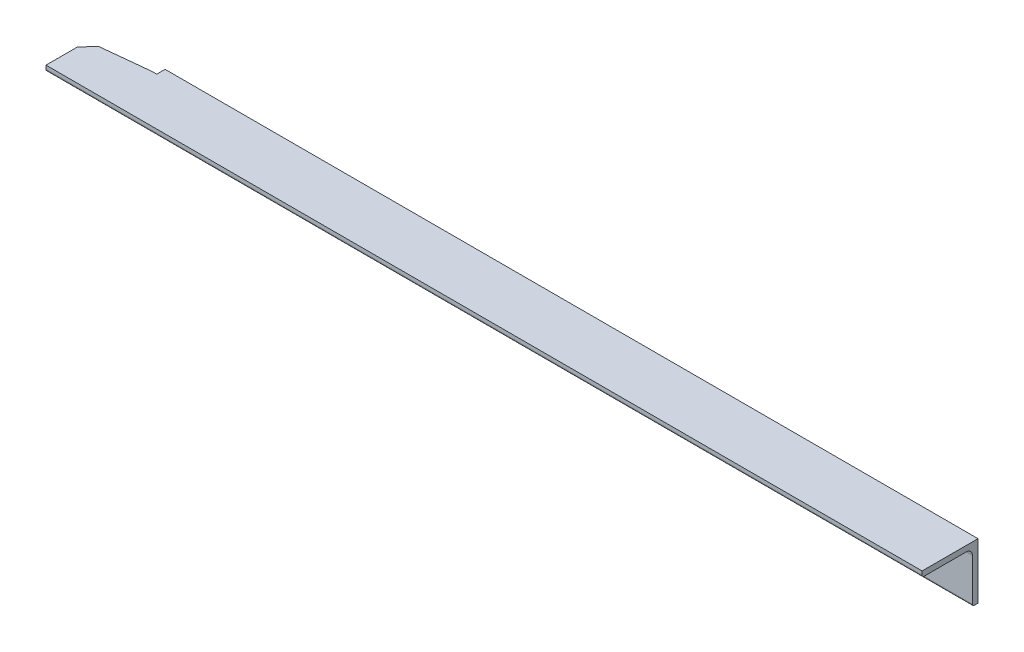
SolidWorks part; units mm, degrees
material "SPCC冷轧板喷塑"
ref_plane "前视基准面" through (0, 0, 0) normal (0, 0, 1) x (1, 0, 0)
ref_plane "上视基准面" through (0, 0, 0) normal (0, 1, 0) x (1, 0, 0)
ref_plane "右视基准面" through (0, 0, 0) normal (1, 0, 0) x (0, 0, -1)
other "Configuration Table"
sketch "草图1" plane through (0, 0, 0) normal (0, 0, 1) x (1, 0, 0)
  line L0 (391.75, 0) -> (-391.75, 0)
  point P4 (0, 0)
  dimension "D1" = 783.5
other "Gbt706-2008 热轧等边角钢 050×5(1)"
ref_plane "基准面1" through (391.75, 0, 0) normal (-1, 0, 0) x (0, -1, 0)
sketch "Sketch1" plane through (391.75, 0, 0) normal (-1, 0, 0) x (0, -1, 0)
  line L0 (0, 0) -> (0, 50)
  line L1 (0, 25) -> (5, 25) construction
  line L2 (5, 48.3333) -> (5, 10.5)
  line L3 (10.5, 5) -> (48.3333, 5)
  line L4 (25, 5) -> (25, 0) construction
  line L5 (50, 0) -> (0, 0)
  line L6 (0, 50) -> (3.3333, 50)
  line L7 (50, 0) -> (50, 3.3333)
  arc A0 (50, 3.3333) -> (48.3333, 5) centre (48.3333, 3.3333) ccw
  arc A1 (3.3333, 50) -> (5, 48.3333) centre (3.3333, 48.3333) cw
  arc A2 (10.5, 5) -> (5, 10.5) centre (10.5, 10.5) cw
  point P10 (25, 0)
  point P14 (0, 25)
  point P15 (5, 25)
  point P16 (25, 5)
  point P17 (5, 50)
  point P18 (50, 5)
  point P21 (50, 5)
  point P24 (5, 50)
  point P25 (0, 0)
sketch "草图2" plane through (0, 0, 0) normal (0, 1, 0) x (1, 0, 0)
  line L0 (-335.25, 0) -> (-335.25, -7.5014)
  line L1 (-391.75, 0) -> (391.75, 0) construction
  line L2 (-335.25, -2.5288) -> (-335.25, 0) construction
  line L3 (-339.7274, -7.5014) -> (-382.7953, -12.028)
  line L4 (-382.7953, -12.028) -> (-391.75, -21.9732)
  line L5 (-391.75, -50) -> (-391.75, 0) construction
  line L6 (-391.75, -21.9732) -> (-382.7953, -12.028) construction
  line L7 (-391.75, -21.9732) -> (-391.75, -52.5014)
  line L8 (-391.75, -138.0268) -> (-391.75, -21.9732) construction
  line L9 (-391.75, -52.5014) -> (-406.75, -52.5014)
  line L10 (-406.75, -52.5014) -> (-406.75, 7.4986)
  line L11 (-406.75, 7.4986) -> (-335.25, 7.4986)
  line L12 (-335.25, 7.4986) -> (-335.25, 0)
  line L13 (-335.25, -7.5014) -> (-339.7274, -7.5014)
  dimension "D1" = 15
  dimension "D2" = 15
  dimension "D3" = 60
extrude "切除-拉伸1" cut sketch "草图2" against normal through all
sketch "草图3" plane through (0, 0, 5) normal (0, 0, 1) x (1, 0, 0)
  line L0 (-25.75, -30) -> (-21.75, -30) construction
  line L1 (-25.75, -25.5) -> (-21.75, -25.5)
  line L2 (-25.75, -34.5) -> (-21.75, -34.5)
  line L3 (-19.25, -27.9801) -> (-19.25, -31.98) construction
  line L4 (-335.25, 0) -> (391.75, 0) construction
  line L5 (-311.75, -30) -> (-307.75, -30) construction
  line L6 (-311.75, -25.5) -> (-307.75, -25.5)
  line L7 (-311.75, -34.5) -> (-307.75, -34.5)
  line L8 (-25.75, -30) -> (-311.75, -30) construction
  arc A0 (-25.75, -25.5) -> (-25.75, -34.5) centre (-25.75, -30) ccw
  arc A1 (-21.75, -34.5) -> (-21.75, -25.5) centre (-21.75, -30) ccw
  arc A2 (-311.75, -25.5) -> (-311.75, -34.5) centre (-311.75, -30) ccw
  arc A3 (-307.75, -34.5) -> (-307.75, -25.5) centre (-307.75, -30) ccw
  point P2 (-23.75, -30)
  point P15 (-309.75, -30)
  dimension "D2" = 13
  dimension "D1" = 9
  dimension "D3" = 4.5
  dimension "D4" = 30
  dimension "D6" = 286
  dimension "D5" = 2
extrude "切除-拉伸2" cut sketch "草图3" against normal up to next
equation "\"D2@Sketch1\"= \"D1@Sketch1\" / 3"
